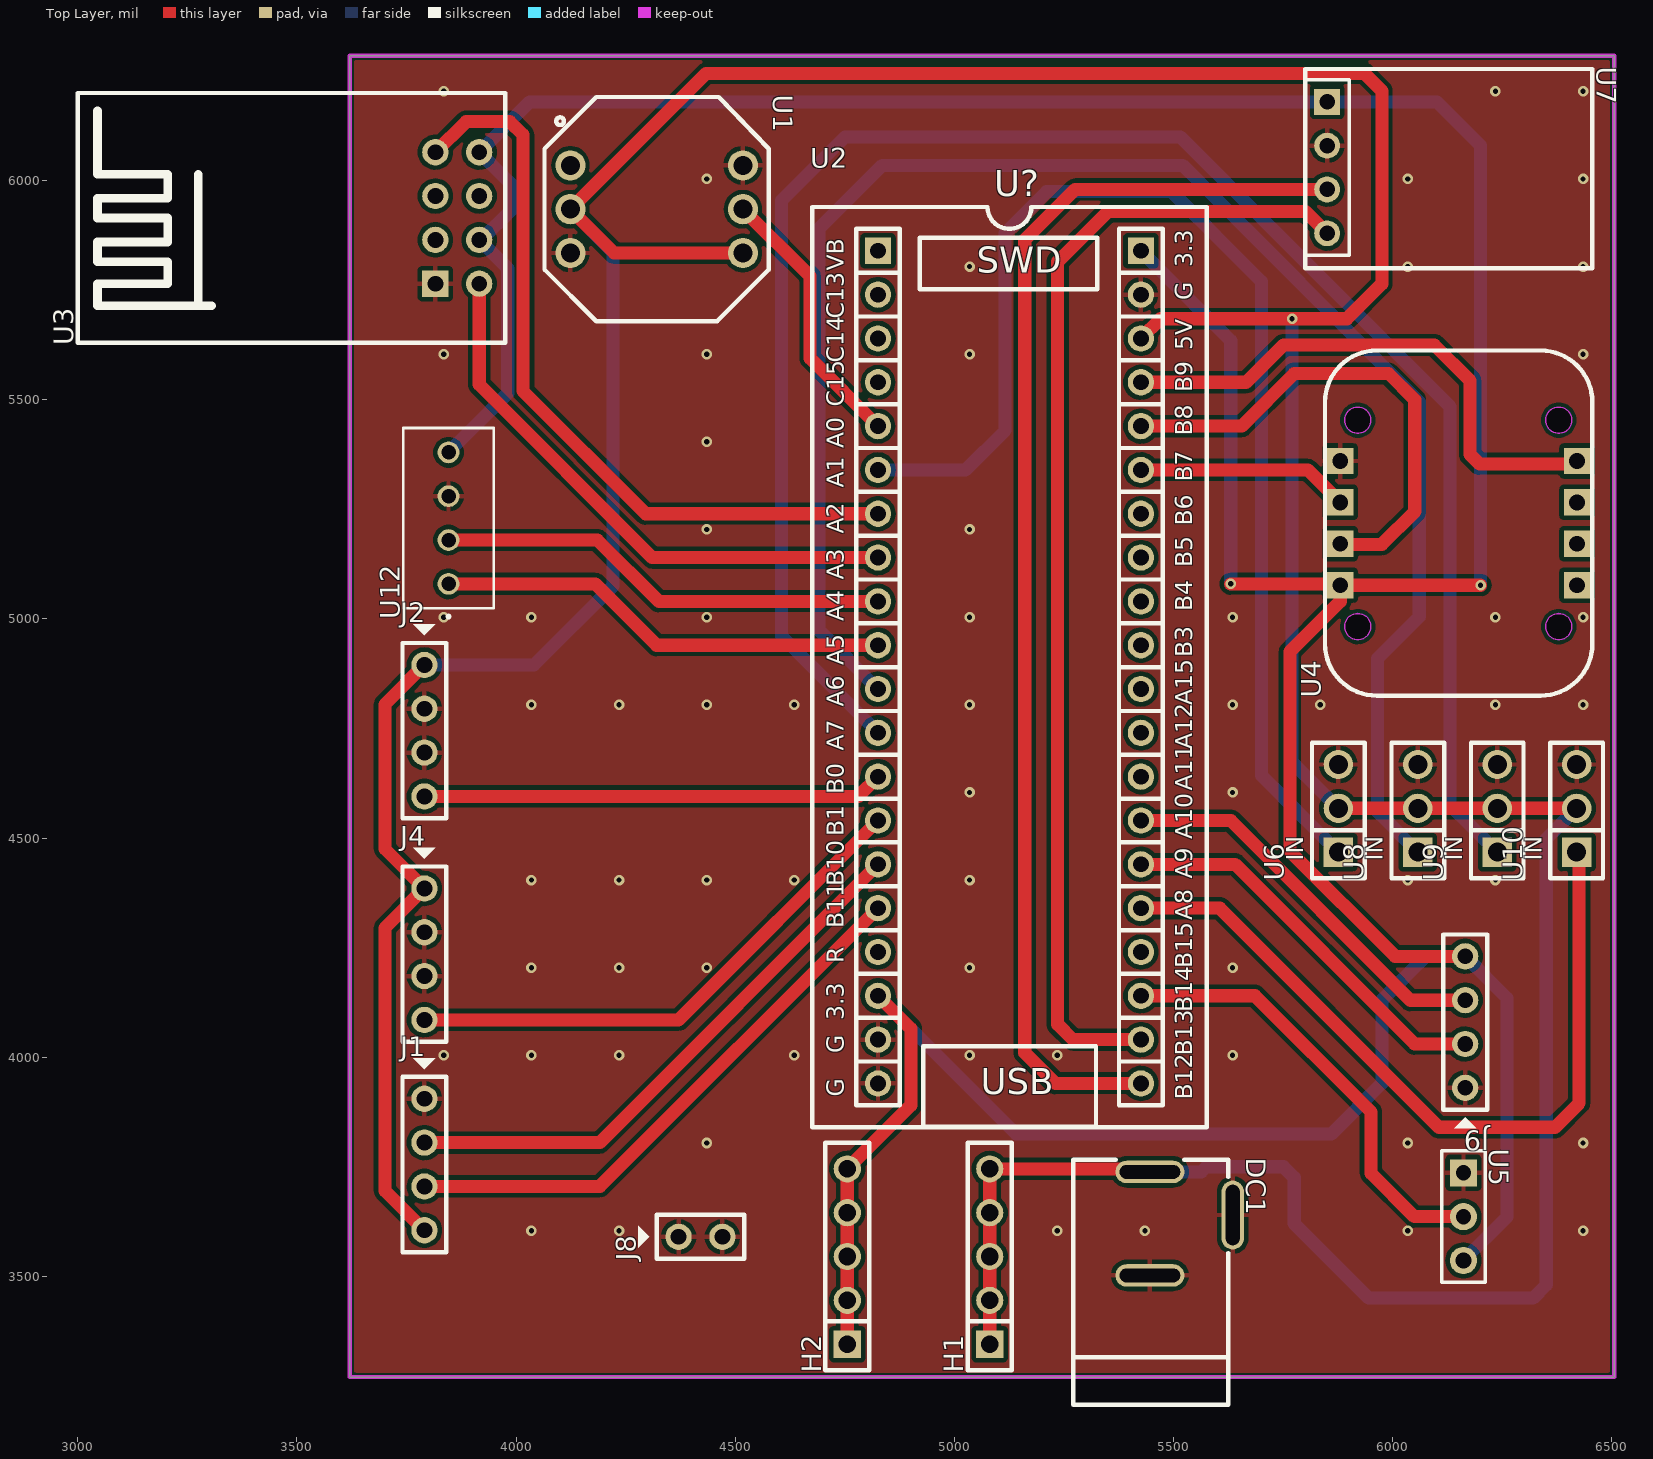
[diagram p0: Top Layer view]
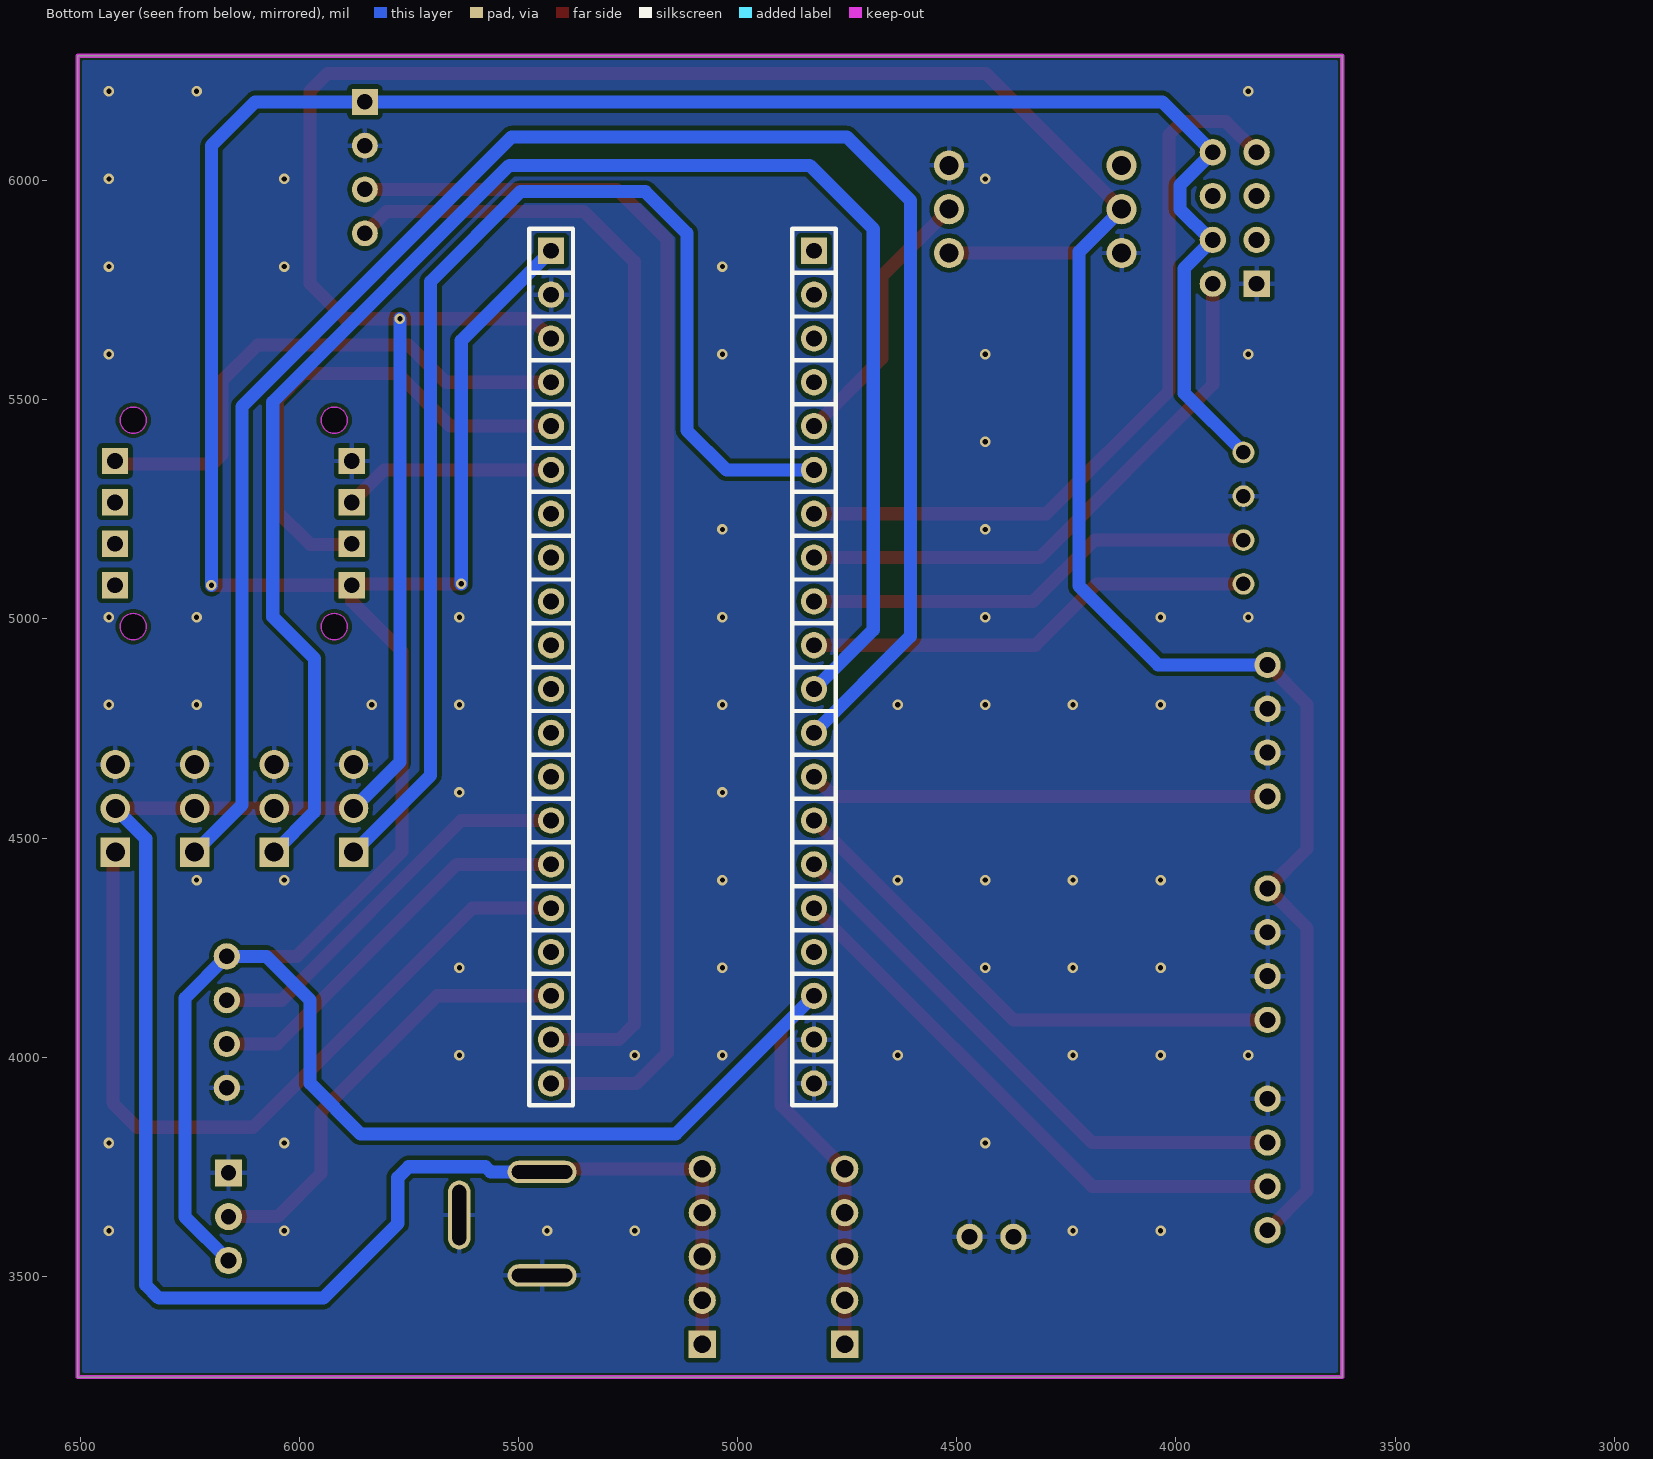
[diagram p1: Bottom Layer view, seen from below]
# Altium PCB MISC51766.pcbdoc
Units mil, origin at the board's own origin, x right, y up, seen from the top; angles counter-clockwise.
Board outline 2885 x 3015 mil, 2 copper layers (Top Layer, Bottom Layer), stack 62.206 mil thick; 19 components, 24 nets, 116 pads, 65 vias.

## Layer stack, top to bottom
Top Solder Mask Layer: solder mask 0.394, Dk 3.3
Top Layer: signal copper 1.379
Dielectric1: surface 59.449, FR4, Dk 4.5
Bottom Layer: signal copper 1.378
Bottom Solder Mask Layer: solder mask 0.394, Dk 3.3

## Board outline
3620.95,6285 3620.95,3270 6505.94,3270 6505.94,6285

## Design rules (kind name [scope] priority, off if disabled: settings)
BoardOutlineClearance copperThickness2oz_1 [All] p2 off: genericclearance=7.99 ignorepadtopadclearanceinfootprint=FALSE except(0: Arc-SplitContinuation Track-SplitContinuation SMDPad-SplitContinuation THPad-SplitContinuation Via-SplitContinuation Fill-SplitContinuation Region-SplitContinuation Poly-SplitContinuation Text-SplitContinuation Hole-SplitContinuation; 5.98: Arc-CutoutEdge SMDPad-CutoutEdge THPad-CutoutEdge Via-CutoutEdge Fill-CutoutEdge Region-CutoutEdge Text-CutoutEdge; 6.93: Hole-OutlineEdge Hole-CutoutEdge; 10: Poly-OutlineEdge Poly-CutoutEdge; 11.81: Arc-OutlineEdge Track-OutlineEdge SMDPad-OutlineEdge THPad-OutlineEdge Via-OutlineEdge Fill-OutlineEdge Region-OutlineEdge Text-OutlineEdge Track-CutoutEdge)
BoardOutlineClearance copperThickness1oz_1 [All] p4: genericclearance=4.02 ignorepadtopadclearanceinfootprint=FALSE except(0: Arc-SplitContinuation Track-SplitContinuation SMDPad-SplitContinuation THPad-SplitContinuation Via-SplitContinuation Fill-SplitContinuation Region-SplitContinuation Poly-SplitContinuation Text-SplitContinuation Hole-SplitContinuation; 6: SMDPad-CutoutEdge THPad-CutoutEdge Via-CutoutEdge Fill-CutoutEdge Region-CutoutEdge Text-CutoutEdge; 6.93: Hole-OutlineEdge Hole-CutoutEdge; 10: Poly-OutlineEdge Poly-CutoutEdge; 11.8: Arc-OutlineEdge Track-OutlineEdge SMDPad-OutlineEdge THPad-OutlineEdge Via-OutlineEdge Fill-OutlineEdge Region-OutlineEdge Text-OutlineEdge; 11.81: Arc-CutoutEdge Track-CutoutEdge)
Clearance copperThickness2oz [All] p1 off: gap=7.99 ignorepadtopadclearanceinfootprint=FALSE except(5.98: SMDPad-Track SMDPad-SMDPad THPad-Track SMDPad-THPad THPad-THPad Track-Via SMDPad-Via THPad-Via Via-Via Fill-Track Region-Track Fill-SMDPad Region-SMDPad Fill-THPad Region-THPad Fill-Via Region-Via Fill-Fill Fill-Region Region-Region Arc-Track Arc-SMDPad Arc-THPad Arc-Via Fill-Arc Region-Arc Arc-Arc Text-Track SMDPad-Text Text-THPad Text-Via Fill-Text Region-Text Arc-Text Text-Text; 6.93: Hole-Track Hole-SMDPad Hole-THPad Hole-Via Fill-Hole Region-Hole Hole-Arc Hole-Text; 10: Poly-Track Poly-SMDPad Poly-THPad Poly-Via Poly-Fill Poly-Region Poly-Poly Poly-Arc Poly-Text Poly-Hole)
Clearance copperThickness1oz [All] p3: gap=4.02 ignorepadtopadclearanceinfootprint=FALSE except(5.98: SMDPad-Track SMDPad-SMDPad THPad-Track SMDPad-THPad THPad-THPad Track-Via SMDPad-Via THPad-Via Via-Via Fill-Track Region-Track Fill-SMDPad Region-SMDPad Fill-THPad Region-THPad Fill-Via Region-Via Fill-Fill Fill-Region Region-Region; 6: Arc-Track Arc-SMDPad Arc-THPad Arc-Via Fill-Arc Region-Arc Arc-Arc Text-Track SMDPad-Text Text-THPad Text-Via Fill-Text Region-Text Arc-Text Text-Text; 6.93: Hole-Track Hole-SMDPad Hole-THPad Hole-Via Fill-Hole Region-Hole Hole-Arc Hole-Text; 10: Poly-Track Poly-SMDPad Poly-THPad Poly-Via Poly-Fill Poly-Region Poly-Poly Poly-Arc Poly-Text Poly-Hole)
DiffPairsRouting differentialPair [All] p1: maxlimit=6 minlimit=6 mostfreqgap=6 toplayer_minwidth=5 toplayer_prefwidth=10 toplayer_maxwidth=100 toplayer_mingap=6 toplayer_prefgap=6 toplayer_maxgap=6 bottomlayer_minwidth=5 bottomlayer_prefwidth=10 bottomlayer_maxwidth=100 bottomlayer_mingap=6 bottomlayer_prefgap=6 bottomlayer_maxgap=6 maxuncoupledlength=10
HoleToHoleClearance otherClearance [All] p1: gap=11.81 allowstackedmicrovias=TRUE
Length netLength [All] p1: minlimit=0 maxlimit=0
MatchedLengths netLengthTolerance [All] p1: tolerance=1000
PasteMaskExpansion pasteMaskExpansion [All] p1: expansion=0
PlaneConnect innerPlane [All] p1: planeconnectstyle=Relief reliefexpansion=20 reliefentries=4 reliefconductorwidth=10 reliefairgap=10
PolygonConnect copperRegion [(InNet('GND'))] p1: connectstyle=Relief reliefconductorwidth=10 reliefentries=4 polygonreliefangle="90 Angle" airgapwidth=10 via.connectstyle=Relief via.reliefconductorwidth=10 via.reliefentries=4 via.polygonreliefangle="90 Angle" via.airgapwidth=10
RoutingVias viaSize [All] p1: holewidth=12.01 width=24.02 viastyle="Through Hole" minholewidth=11.81 minwidth=19.68 maxholewidth=248.03 maxwidth=393.7
SolderMaskExpansion solderMaskExpansion [IsVia] p1: expansion=-1000 istentingtop=TRUE
SolderMaskExpansion solderMaskExpansion [All] p2: expansion=2 istentingtop=FALSE
Width copperThickness2oz_2 [All] p1 off: maxlimit=100 minlimit=8 preferedwidth=10
Width copperThickness1oz_2 [All] p2: maxlimit=100 minlimit=5 preferedwidth=10

## Components (designator, comment, footprint, x,y, rotation, side; value= is the part's Value field where it differs from the comment)
DC1 "" DC-2.0 5435.94,3615 r270 top
H1 "" HDR-TH_5P-P2.54-V-F 5080.94,3545 r90 top
H2 "" HDR-TH_5P-P2.54-V-F 4755.94,3545 r90 top
J1 "HDR-TH_4P-2.54MM" HDR-TH_4P-2.54MM 3790.95,3905 r0 top
J2 "HDR-TH_4P-2.54MM" HDR-TH_4P-2.54MM 3790.95,4895 r0 top
J4 "HDR-TH_4P-2.54MM" HDR-TH_4P-2.54MM 3790.95,4385 r0 top
J8 "HDR-TH_2P-2.54MM" HDR-TH_2P-2.54MM 4370.94,3590 r90 top
J9 "HDR-TH_4P-2.54MM" HDR-TH_4P-2.54MM 6165.94,3930 r180 top
U1 "XGZP6847A" SENSOR-TH_XGZP6847A 4320.94,5935 r270 top
U2 "STM32C8T6 minimum system" STM32F103C8T6最小系统插座 4725.94,5940 r0 top
U3 "ESP8266-01S" WIFIM-TH_ESP8266-01S 3865.95,5915 r90 top
U4 "MAX30102" MAX30102 5845.94,4825 r90 top
U5 "MH-FMD" MH-FMD 6155.94,3625 r270 top
U6 "SG90 servo - back (0-90)" SG90 5876.42,4567.81 r90 top
U7 "GY-906-DCC" GY-906-DCC 6155.94,6040 r270 top
U8 "SG90 servo - leg (0-90)" SG90 6057.77,4567.81 r90 top
U9 "SG90 servo - left flip (0-30)" SG90 6239.12,4567.81 r90 top
U10 "SG90 servo - right flip (0-30)" SG90 6420.47,4567.81 r90 top
U12 "" SHT30 3845.95,5080 r90 top

## Footprints (in the part's own frame and the unit in brackets; to place one, negate y for a bottom-side part, rotate by r counter-clockwise, add the part's x,y. Pads: shape width x height; smd on the part's side, far side on the other; paste and mask are expansions set on the pad)
DC-2.0 [mil]
  oval 157.5x51.2 hole 31.5 slot 137.8 at 0 deg paste+0 mask+2: 2(-24.7,199.5)
  oval 51.2x157.5 hole 31.5 slot 137.8 at 90 deg paste+0 mask+2: 3(113.1,10.5) 4(-123.1,10.5)
  silkscreen extent -151,-165 408,190
GY-906-DCC [mil]
  rect 59.05x59.05 hole 35.43 paste+0 mask+2: 1(-140,-305)
  round 59.05 hole 35.43 paste+0 mask+2: 2(-40,-305) 3(60,-305) 4(160,-305)
  silkscreen extent -215,-355 240,300
HDR-TH_2P-2.54MM [mil]
  round 60 hole 36 paste+0 mask+4: 1(0,0) 2(0,-100)
  silkscreen extent -50,-150 50,92
HDR-TH_4P-2.54MM [mil]
  round 60 hole 36 paste+0 mask+4: 1(0,0) 2(0,-100) 3(0,-200) 4(0,-300)
  silkscreen extent -50,-350 50,92
HDR-TH_5P-P2.54-V-F [mil]
  rect 62x62 hole 40.16: 1(-200,0)
  round 62 hole 40.16: 2(-100,0) 3(0,0) 4(100,0) 5(200,0)
  silkscreen extent -260,-50 260,50
MAX30102 [mil]
  rect 60x60 hole 36: 1(251.97,-35) 2(346.46,-35) 3(440.94,-35) 4(535.43,-35) 5(251.97,-575) 6(346.46,-575) 7(440.94,-575) 8(535.43,-575)
  Board Outline Layer circle w0.1: c157.48,-74.8 r30
  Board Outline Layer circle w0.1: c157.48,-533.46 r30
  Board Outline Layer circle w0.1: c628.5,-74.8 r30
  Board Outline Layer circle w0.1: c628.5,-533.46 r30
  Board Outline Layer region: 157.48,-104.8 144.46,-101.83 134.03,-93.51 128.23,-81.48 128.23,-68.13 134.03,-56.1 144.46,-47.77 157.48,-44.8 157.48,-44.8 170.5,-47.77 180.94,-56.1 186.73,-68.13 186.73,-81.48 180.94,-93.51 170.5,-101.83 157.48,-104.8
  Board Outline Layer region: 157.48,-104.8 152.79,-104.43 148.21,-103.33 143.86,-101.53 139.85,-99.07 136.27,-96.02 133.21,-92.44 130.75,-88.42 128.95,-84.07 127.85,-79.5 127.48,-74.8 127.85,-70.11 128.95,-65.53 130.75,-61.18 133.21,-57.17 136.27,-53.59 139.85,-50.53 143.86,-48.07 148.21,-46.27 152.79,-45.17 157.48,-44.8 162.17,-45.17 166.75,-46.27 171.1,-48.07 175.11,-50.53 178.69,-53.59 181.75,-57.17 184.21,-61.18 186.01,-65.53 187.11,-70.11 187.48,-74.8 187.11,-79.5 186.01,-84.07 184.21,-88.42 181.75,-92.44 178.69,-96.02 175.11,-99.07 171.1,-101.53 166.75,-103.33 162.17,-104.43
  Board Outline Layer region: 157.48,-563.46 144.46,-560.49 134.03,-552.17 128.23,-540.14 128.23,-526.79 134.03,-514.76 144.46,-506.44 157.48,-503.46 157.48,-503.46 170.5,-506.44 180.94,-514.76 186.73,-526.79 186.73,-540.14 180.94,-552.17 170.5,-560.49 157.48,-563.46
  Board Outline Layer region: 157.48,-563.46 152.79,-563.1 148.21,-562 143.86,-560.19 139.85,-557.74 136.27,-554.68 133.21,-551.1 130.75,-547.08 128.95,-542.74 127.85,-538.16 127.48,-533.46 127.85,-528.77 128.95,-524.19 130.75,-519.84 133.21,-515.83 136.27,-512.25 139.85,-509.19 143.86,-506.73 148.21,-504.93 152.79,-503.83 157.48,-503.46 162.17,-503.83 166.75,-504.93 171.1,-506.73 175.11,-509.19 178.69,-512.25 181.75,-515.83 184.21,-519.84 186.01,-524.19 187.11,-528.77 187.48,-533.46 187.11,-538.16 186.01,-542.74 184.21,-547.08 181.75,-551.1 178.69,-554.68 175.11,-557.74 171.1,-560.19 166.75,-562 162.17,-563.1
  Board Outline Layer region: 628.5,-104.8 615.49,-101.83 605.05,-93.51 599.26,-81.48 599.26,-68.13 605.05,-56.1 615.49,-47.77 628.5,-44.8 628.5,-44.8 641.52,-47.77 651.96,-56.1 657.75,-68.13 657.75,-81.48 651.96,-93.51 641.52,-101.83 628.5,-104.8
  Board Outline Layer region: 628.5,-104.8 623.81,-104.43 619.23,-103.33 614.88,-101.53 610.87,-99.07 607.29,-96.02 604.23,-92.44 601.77,-88.42 599.97,-84.07 598.87,-79.5 598.5,-74.8 598.87,-70.11 599.97,-65.53 601.77,-61.18 604.23,-57.17 607.29,-53.59 610.87,-50.53 614.88,-48.07 619.23,-46.27 623.81,-45.17 628.5,-44.8 633.2,-45.17 637.77,-46.27 642.12,-48.07 646.14,-50.53 649.72,-53.59 652.77,-57.17 655.23,-61.18 657.04,-65.53 658.13,-70.11 658.5,-74.8 658.13,-79.5 657.04,-84.07 655.23,-88.42 652.77,-92.44 649.72,-96.02 646.14,-99.07 642.12,-101.53 637.77,-103.33 633.2,-104.43
  Board Outline Layer region: 628.5,-563.46 615.49,-560.49 605.05,-552.17 599.26,-540.14 599.26,-526.79 605.05,-514.76 615.49,-506.44 628.5,-503.46 628.5,-503.46 641.52,-506.44 651.96,-514.76 657.75,-526.79 657.75,-540.14 651.96,-552.17 641.52,-560.49 628.5,-563.46
  Board Outline Layer region: 628.5,-563.46 623.81,-563.1 619.23,-562 614.88,-560.19 610.87,-557.74 607.29,-554.68 604.23,-551.1 601.77,-547.08 599.97,-542.74 598.87,-538.16 598.5,-533.46 598.87,-528.77 599.97,-524.19 601.77,-519.84 604.23,-515.83 607.29,-512.25 610.87,-509.19 614.88,-506.73 619.23,-504.93 623.81,-503.83 628.5,-503.46 633.2,-503.83 637.77,-504.93 642.12,-506.73 646.14,-509.19 649.72,-512.25 652.77,-515.83 655.23,-519.84 657.04,-524.19 658.13,-528.77 658.5,-533.46 658.13,-538.16 657.04,-542.74 655.23,-547.08 652.77,-551.1 649.72,-554.68 646.14,-557.74 642.12,-560.19 637.77,-562 633.2,-563.1
  Multi-Layer board cut-out: 157.48,-104.8 144.46,-101.83 134.03,-93.51 128.23,-81.48 128.23,-68.13 134.03,-56.1 144.46,-47.77 157.48,-44.8 157.48,-44.8 170.5,-47.77 180.94,-56.1 186.73,-68.13 186.73,-81.48 180.94,-93.51 170.5,-101.83 157.48,-104.8
  Multi-Layer board cut-out: 157.48,-563.46 144.46,-560.49 134.03,-552.17 128.23,-540.14 128.23,-526.79 134.03,-514.76 144.46,-506.44 157.48,-503.46 157.48,-503.46 170.5,-506.44 180.94,-514.76 186.73,-526.79 186.73,-540.14 180.94,-552.17 170.5,-560.49 157.48,-563.46
  Multi-Layer board cut-out: 628.5,-104.8 615.49,-101.83 605.05,-93.51 599.26,-81.48 599.26,-68.13 605.05,-56.1 615.49,-47.77 628.5,-44.8 628.5,-44.8 641.52,-47.77 651.96,-56.1 657.75,-68.13 657.75,-81.48 651.96,-93.51 641.52,-101.83 628.5,-104.8
  Multi-Layer board cut-out: 628.5,-563.46 615.49,-560.49 605.05,-552.17 599.26,-540.14 599.26,-526.79 605.05,-514.76 615.49,-506.44 628.5,-503.46 628.5,-503.46 641.52,-506.44 651.96,-514.76 657.75,-526.79 657.75,-540.14 651.96,-552.17 641.52,-560.49 628.5,-563.46
  silkscreen extent 0,-610 787,0
MH-FMD [mil]
  rect 62x62 hole 35 paste+0 mask+2: 1(-111,6)
  round 62 hole 35 paste+0 mask+2: 2(-11,6)
  round 62 hole 36 paste+0 mask+2: 3(89,6)
  silkscreen extent -161,-43 139,56
SENSOR-TH_XGZP6847A [mm]
  round 1.75 hole 1.1 paste+0 mask+0.05: 1(-2.54,-5) 2(0,-5) 3(2.54,-5) 4(2.54,5) 5(0,5) 6(-2.54,5)
  silkscreen extent -6.5,-6.5 6.5,6.5
SG90 [mm]
  rect 1.7x1.7 hole 1.1 paste+0 mask+0.051: 1(-2.54,0)
  round 1.7 hole 1.1 paste+0 mask+0.051: 2(0,0) 3(2.54,0)
  silkscreen extent -4.06,-1.52 3.81,1.52
SHT30 [mil]
  round 49.61 hole 33.07 paste+0 mask+2: 1(0,0) 2(100,0) 3(200,0) 4(300,0)
  silkscreen extent -81,-103 356,103
STM32F103C8T6最小系统插座 [mil]
  rect 60x60 hole 36 paste+0 mask+2: 1(100,-100) 40(700,-100)
  round 60 hole 36 paste+0 mask+2: 2(100,-200) 3(100,-300) 4(100,-400) 5(100,-500) 6(100,-600) 7(100,-700) 8(100,-800) 9(100,-900) 10(100,-1000) 11(100,-1100) 12(100,-1200) 13(100,-1300) 14(100,-1400) 15(100,-1500) 16(100,-1600) 17(100,-1700) 18(100,-1800) 19(100,-1900) 20(100,-2000) 21(700,-2000) 22(700,-1900) 23(700,-1800) 24(700,-1700) 25(700,-1600) 26(700,-1500) 27(700,-1400) 28(700,-1300) 29(700,-1200) 30(700,-1100) 31(700,-1000) 32(700,-900) 33(700,-800) 34(700,-700) 35(700,-600) 36(700,-500) 37(700,-400) 38(700,-300) 39(700,-200)
  silkscreen extent -50,-2100 850,0
WIFIM-TH_ESP8266-01S [mil]
  rect 60x60 hole 36 paste+0 mask+1.97: 1(-150,50)
  round 60 hole 36 paste+0 mask+1.97: 2(-50,50) 3(50,50) 4(150,50) 5(-150,-50) 6(-50,-50) 7(50,-50) 8(150,-50)
  silkscreen extent -285,-109 285,866

## Via types
v1: diameter 24.02, hole 12, Top Layer to Bottom Layer, 65 vias

## Nets (pads, with @x,y where several pads share a name; then routed paths per layer and width w, separated by ;. In a path a pad name is that pad's centre, name@x,y a point inside that pad or via, vN(x,y) a via of type N, cw(c..) or ccw(c..) an arc to the next point about the centre after c; other vN are vias at no path point)
3.3V: H2.1 H2.2 H2.3 H2.4 H2.5 J9.4 U2.18 U2.40 U3.6 U3.8 U4.1 U5.3 U7.1 U12.4 | length 10190.2
  Top Layer w30: H2.1 H2.2 H2.3 H2.4 H2.5 4900.94,3890 4900.94,4065 U2.18 ; v1(5630.94,5080) 5877.91,5080 U4.1 ; J9.4 6005.94,4230 5765.94,4470 5765.94,4925 5880.94,5040 U4.1 ; v1(6200.94,5076.97) U4.1
  Bottom Layer w30: U12.4 3980.95,5515 3980.95,5800 U3.6 3920.95,5865 3990.95,5935 3990.95,5990 U3.8 4030.95,6180 U7.1 6100.94,6180 6200.94,6080 v1(6200.94,5076.97) ; U2.18 5140.94,3825 5860.94,3825 5975.94,3940 5975.94,4130 6075.94,4230 J9.4 6260.94,4135 6260.94,3635 U5.3 ; U2.40 5630.94,5635 v1(5630.94,5080)
5V: DC1.4 H1.1 H1.2 H1.3 H1.4 H1.5 J1.4 J2.1 J4.1 U1.2 U1.4 U2.38 U6.2 U8.2 U9.2 U10.2 | length 11015
  Top Layer w30: J1.4 3700.95,3695 3700.95,4295 J4.1 3700.95,4475 3700.95,4805 J2.1 ; U1.4 4224.1,5835 U1.2 4434.1,6245 5935.94,6245 5975.94,6205 5975.94,5765 5895.94,5685 v1(5770.94,5685) 5470.94,5685 U2.38 ; H1.1 H1.2 H1.3 H1.4 H1.5 5439.55,3745 DC1.4 ; U6.2 U8.2 U9.2 U10.2
  Bottom Layer w30: J2.1 4040.95,4895 4220.94,5075 4220.94,5838.15 U1.2 ; DC1.4 5564.05,3738.1 5575.94,3750 5750.94,3750 5775.94,3725 5775.94,3620 5945.94,3450 6320.94,3450 6350.94,3480 6350.94,4498.29 U10.2 ; v1(5770.94,5685) 5770.94,4673.29 U6.2
GND: DC1.2 DC1.3 J1.1 J2.2 J2.3 J4.2 J4.3 J8.1 J8.2 J9.1 U1.3 U1.6 U2.19 U2.20 U2.39 U3.1 U4.4 U5.1 U6.3 U7.2 U8.3 U9.3 U10.3 U12.3
  other v1: 4035.05,3604.1 4235.05,3604.1 5235.05,3604.1 5435.05,3604.1 6035.05,3604.1 6435.05,3604.1 4435.05,3804.1 6035.05,3804.1 6435.05,3804.1 3835.05,4004.1 4035.05,4004.1 4235.05,4004.1 4635.05,4004.1 5035.05,4004.1 5235.05,4004.1 5635.05,4004.1 4035.05,4204.1 4235.05,4204.1 4435.05,4204.1 5035.05,4204.1 5635.05,4204.1 4035.05,4404.1 4235.05,4404.1 4435.05,4404.1 4635.05,4404.1 5035.05,4404.1 6035.05,4404.1 6235.05,4404.1 5035.05,4604.1 5635.05,4604.1 4035.05,4804.1 4235.05,4804.1 4435.05,4804.1 4635.05,4804.1 5035.05,4804.1 5635.05,4804.1 5835.05,4804.1 6235.05,4804.1 6435.05,4804.1 3835.05,5004.1 4035.05,5004.1 4435.05,5004.1 5035.05,5004.1 5635.05,5004.1 6235.05,5004.1 6435.05,5004.1 4435.05,5204.1 5035.05,5204.1 4435.05,5404.1 3835.05,5604.1 4435.05,5604.1 5035.05,5604.1 6435.05,5604.1 5035.05,5804.1 6035.05,5804.1 6435.05,5804.1 4435.05,6004.1 6035.05,6004.1 6435.05,6004.1 3835.05,6204.1 6235.05,6204.1 6435.05,6204.1
PA0: U1.5 U2.5 | length 622.6
  Top Layer w30: U1.5 4670.94,5781.85 4670.94,5595 U2.5
PA1: U2.6 U6.1 | length 2861.4
  Bottom Layer w30: U2.6 5025.94,5340 5115.94,5430 5115.94,5880 5210.94,5975 5495.94,5975 5700.94,5770 5700.94,4643.29 U6.1
PA2-2TX: U2.7 U3.4 | length 1752.4
  Top Layer w30: U3.4 3885.95,6135 3985.95,6135 4015.95,6105 4015.95,5520 4295.94,5240 U2.7
PA3-2RX: U2.8 U3.5 | length 1303.6
  Top Layer w30: U3.5 3915.94,5535 4310.94,5140 U2.8
PA4: U2.9 U12.2 | length 1038
  Top Layer w30: U12.2 4185.94,5180 4325.94,5040 U2.9
PA5: U2.10 U12.1 | length 1038
  Top Layer w30: U12.1 4180.94,5080 4320.94,4940 U2.10
PA6: U2.11 U8.1 | length 3864.2
  Bottom Layer w30: U2.11 4690.94,4975 4690.94,5890 4835.94,6035 5520.94,6035 6060.94,5495 6060.94,5005 5965.94,4910 5965.94,4559.64 U8.1
PA7: U2.12 U9.1 | length 4207.9
  Bottom Layer w30: U2.12 4605.94,4960 4605.94,5955 4750.94,6100 5515.94,6100 6130.94,5485 6130.94,4575.99 U9.1
PA8: U2.25 U10.1 | length 1805
  Top Layer w30: U2.25 5605.94,4340 6105.94,3840 6370.94,3840 6425.94,3895 6425.94,4462.34 U10.1
PA9: J9.2 U2.26 | length 909.8
  Top Layer w30: U2.26 5640.94,4440 6050.94,4030 J9.2
PA10: J9.3 U2.27 | length 909.8
  Top Layer w30: U2.27 5630.94,4540 6040.94,4130 J9.3
PB0: J2.4 U2.13 | length 1053.6
  Top Layer w30: J2.4 4780.94,4595 U2.13
PB1: J4.4 U2.14 | length 1223.5
  Top Layer w30: J4.4 4370.94,4085 U2.14
PB7: U2.35 U4.3 | length 485.7
  Top Layer w30: U2.35 5806.89,5340 U4.3
PB8: U2.36 U4.2 | length 1156.2
  Top Layer w30: U2.36 5655.94,5440 5775.94,5560 5990.94,5560 6050.94,5500 6050.94,5245 5975.94,5170 5882.4,5170 U4.2
PB9: U2.37 U4.8 | length 1244.2
  Top Layer w30: U2.37 5665.94,5540 5750.94,5625 6095.94,5625 6177.16,5543.79 6177.16,5375 6198.37,5353.79 6414.3,5353.79 U4.8
PB10: J1.2 U2.15 | length 1298
  Top Layer w30: J1.2 4190.94,3805 U2.15
PB11: J1.3 U2.16 | length 1298
  Top Layer w30: J1.3 4190.94,3705 U2.16
PB12: U2.21 U7.3 | length 2886.6
  Top Layer w30: U2.21 5230.94,3940 5160.94,4010 5160.94,5865 5275.94,5980 U7.3
PB13: U2.22 U7.4 | length 2627.8
  Top Layer w30: U2.22 5270.94,4040 5235.94,4075 5235.94,5815 5350.94,5930 5800.94,5930 U7.4
PB14: U2.23 U5.2 | length 1026.8
  Top Layer w30: U2.23 5685.94,4140 5950.94,3875 5950.94,3735 6049.94,3636 U5.2
pads on no net: U1.1 U2.1 U2.2 U2.3 U2.4 U2.17 U2.24 U2.28 U2.29 U2.30 U2.31 U2.32 U2.33 U2.34 U3.2 U3.3 U3.7 U4.5 U4.6 U4.7

## Polygon pours and split planes (outlines as drawn)
GND on Top Layer (solid, remove dead copper, pour order 0): 3380.95,6550 3380.95,3000 6965.94,3000 6965.94,6550
GND on Bottom Layer (solid, remove dead copper, pour order 2): 3455.95,6455 3455.95,3225 6730.94,3225 6730.94,6455

## Keep-outs
Board Outline Layer:
  the board outline again, w10